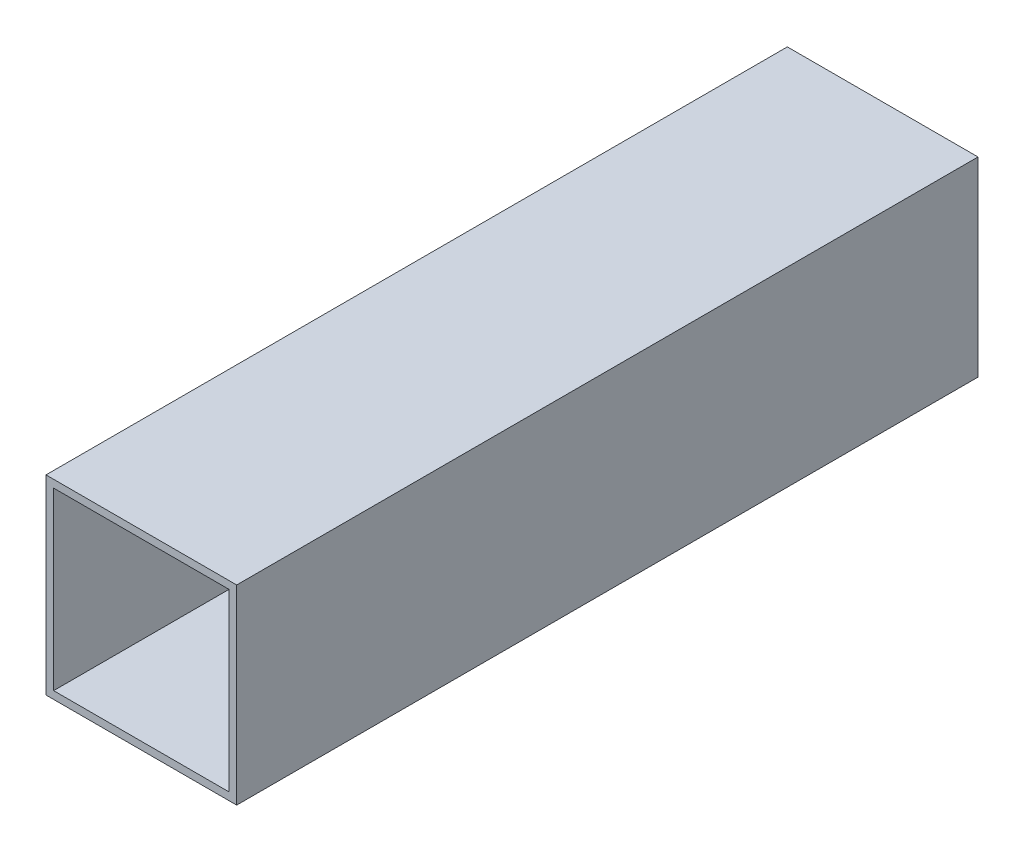
SolidWorks part; units mm, degrees
material "AISI 304"
ref_plane "Front Plane" through (0, 0, 0) normal (0, 0, 1) x (1, 0, 0)
ref_plane "Top Plane" through (0, 0, 0) normal (0, 1, 0) x (1, 0, 0)
ref_plane "Right Plane" through (0, 0, 0) normal (1, 0, 0) x (0, 0, -1)
sketch "Sketch1" plane through (0, 0, 0) normal (0, 0, 1) x (1, 0, 0)
  line L1 (-25, -25) -> (25, -25)
  line L2 (-25, -25) -> (-25, 25)
  line L3 (-25, 25) -> (25, 25)
  line L4 (25, -25) -> (25, 25)
  line L5 (-25, -25) -> (25, 25) construction
  line L6 (-25, 25) -> (25, -25) construction
  line L7 (-23, -23) -> (23, -23)
  line L8 (-23, -23) -> (-23, 23)
  line L9 (-23, 23) -> (23, 23)
  line L10 (23, -23) -> (23, 23)
  line L11 (-23, -23) -> (23, 23) construction
  line L12 (-23, 23) -> (23, -23) construction
  point P0 (0, 0)
  point P6 (0, 0)
  dimension "D1" = 50
  dimension "D2" = 50
  dimension "D3" = 46
  dimension "D4" = 46
extrude "Boss-Extrude1" add sketch "Sketch1" along normal blind 194.4
